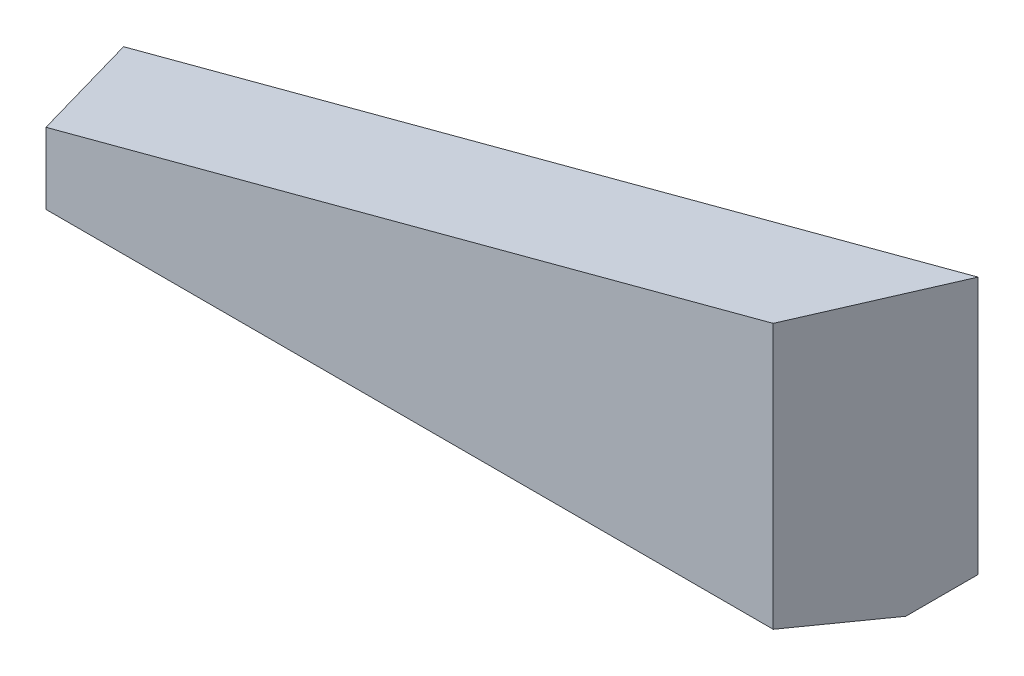
SolidWorks part; units mm, degrees
ref_plane "Front Plane" through (0, 0, 0) normal (0, 0, 1) x (1, 0, 0)
ref_plane "Top Plane" through (0, 0, 0) normal (0, 1, 0) x (1, 0, 0)
ref_plane "Right Plane" through (0, 0, 0) normal (1, 0, 0) x (0, 0, -1)
sketch "Sketch1" plane through (0, 0, 0) normal (0, 0, 1) x (1, 0, 0)
  line L0 (5, 0) -> (137.6, 0)
  line L1 (142.6, 5) -> (142.6, 48)
  line L2 (142.6, 48) -> (0, 10)
  line L3 (0, 10) -> (0, 5)
  line L4 (0, 5) -> (5, 0)
  line L5 (137.6, 0) -> (142.6, 5)
  point P0 (0, 0)
  point P1 (142.6, 0)
  dimension "D1" = 10
  dimension "D2" = 48
  dimension "D3" = 142.6
extrude "Boss-Extrude1" add sketch "Sketch1" along normal blind 20
sketch "Sketch2" plane through (-2.4881, 9.337, 0) normal (-0.2575, 0.9663, 0) x (0.9663, 0.2575, 0)
  line L0 (150.1512, 0) -> (135.4749, -20)
  line L2 (150.1512, -20) -> (135.4749, -20)
  line L3 (150.1512, -20) -> (150.1512, 0) construction
  line L4 (150.1512, -20) -> (150.1512, 0)
  line L5 (2.5749, -20) -> (2.5749, 0) construction
  line L6 (2.5749, -20) -> (2.5749, 0)
  line L7 (9.8749, -20) -> (2.5749, -20)
  line L9 (2.5749, 0) -> (9.8749, -20)
  line L10 (150.1512, -20) -> (2.5749, -20) construction
  dimension "D3" = 7.3
  dimension "D4" = 125.6
extrude "Cut-Extrude1" cut sketch "Sketch2" along direction (0, 1, 0) on the side against the normal blind 50
